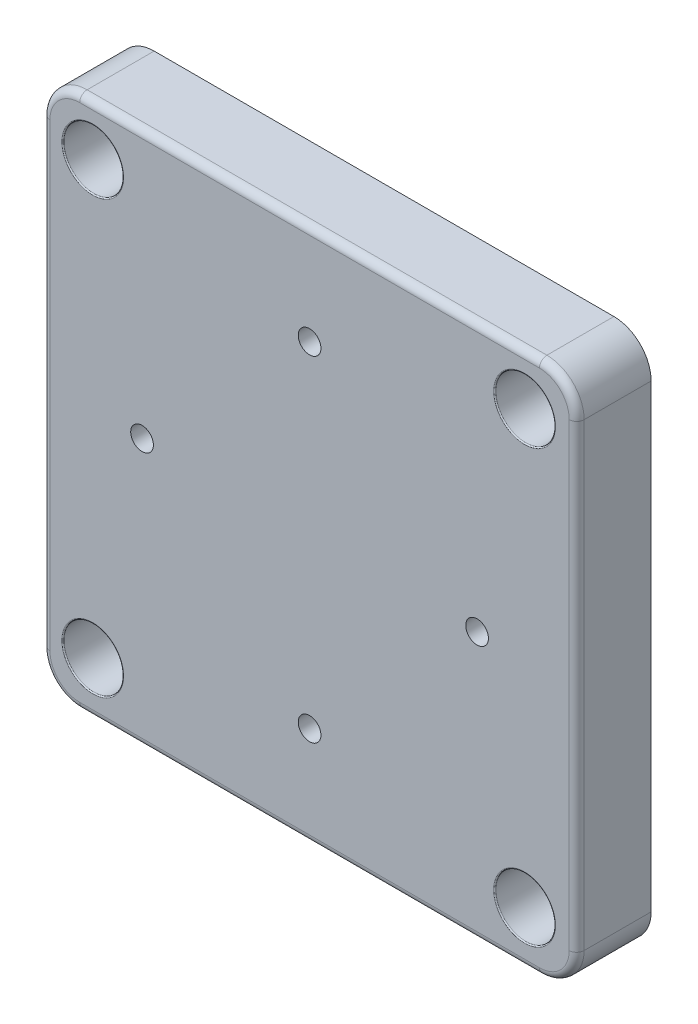
SolidWorks part; units mm, degrees
material "1060 Сплав"
ref_plane "Front" through (0, 0, 0) normal (0, 0, 1) x (1, 0, 0)
ref_plane "Top" through (0, 0, 0) normal (0, 1, 0) x (1, 0, 0)
ref_plane "Right" through (0, 0, 0) normal (1, 0, 0) x (0, 0, -1)
sketch "Sketch1" plane through (0, 0, 0) normal (0, 0, 1) x (1, 0, 0)
  line L0 (0, -35.875) -> (0, 35.875) construction
  line L1 (-35.875, 35.875) -> (35.875, 35.875)
  line L2 (-35.875, 35.875) -> (-35.875, -35.875)
  line L3 (-35.875, -35.875) -> (35.875, -35.875)
  line L4 (35.875, 35.875) -> (35.875, -35.875)
  line L12 (28.875, 29.125) -> (-29.125, 29.125) construction
  line L13 (-29.125, 29.125) -> (-29.125, -28.875) construction
  line L14 (-25.125, -28.875) -> (24.875, -28.875) construction
  line L15 (28.875, -24.875) -> (28.875, 25.125) construction
  line L16 (28.875, -32.875) -> (28.875, -35.875) construction
  line L17 (32.875, -28.875) -> (35.875, -28.875) construction
  line L18 (-29.125, 33.125) -> (-29.125, 35.875) construction
  line L19 (-33.125, 29.125) -> (-35.875, 29.125) construction
  circle A0 centre (-29.125, 29.125) radius 4
  circle A1 centre (28.875, 29.125) radius 4
  circle A2 centre (28.875, -28.875) radius 4
  circle A3 centre (-29.125, -28.875) radius 4
  point P25 (0, 0)
  dimension "D1" = 8
  dimension "D6" = 8
  dimension "D7" = 8
  dimension "D8" = 8
  dimension "D9" = 50
  dimension "D2" = 71.75
  dimension "D3" = 71.75
  dimension "D10" = 50
  dimension "D11" = 3
  dimension "D12" = 3
extrude "Boss-Extrude1" add sketch "Sketch1" along normal blind 10
fillet "Fillet1" radius 5 4 edges at (35.875, -35.875, 5) (-35.875, -35.875, 5) (35.875, 35.875, 5) (-35.875, 35.875, 5)
fillet "Fillet2" radius 1 8 edges at (0, -35.875, 10) (34.4105, -34.4105, 10) (-34.4105, -34.4105, 10) (35.875, 0, 10) (34.4105, 34.4105, 10) (0, 35.875, 10) (-34.4105, 34.4105, 10) (-35.875, 0, 10)
fillet "Fillet4" radius 0.15 4 edges at (32.875, -28.875, 10) (-25.125, -28.875, 10) (-25.125, 29.125, 10) (32.875, 29.125, 10)
sketch "Sketch2" plane through (0, 0, 10) normal (0, 0, 1) x (1, 0, 0)
  line L0 (0, 34.875) -> (0, -34.875) construction
  line L1 (30.875, 34.875) -> (-30.875, 34.875) construction
  line L2 (-30.875, -34.875) -> (30.875, -34.875) construction
  circle A0 centre (0, 0) radius 22.5 construction
  circle A1 centre (0, 22.5) radius 1.525
  circle A2 centre (22.5, 0) radius 1.525
  circle A3 centre (0, -22.5) radius 1.525
  circle A4 centre (-22.5, 0) radius 1.525
  point P19 (0, 0)
  dimension "D1" = 45
  dimension "D2" = 3.05
  dimension "D3" = 4
extrude "Cut-Extrude1" cut sketch "Sketch2" against normal blind 10
